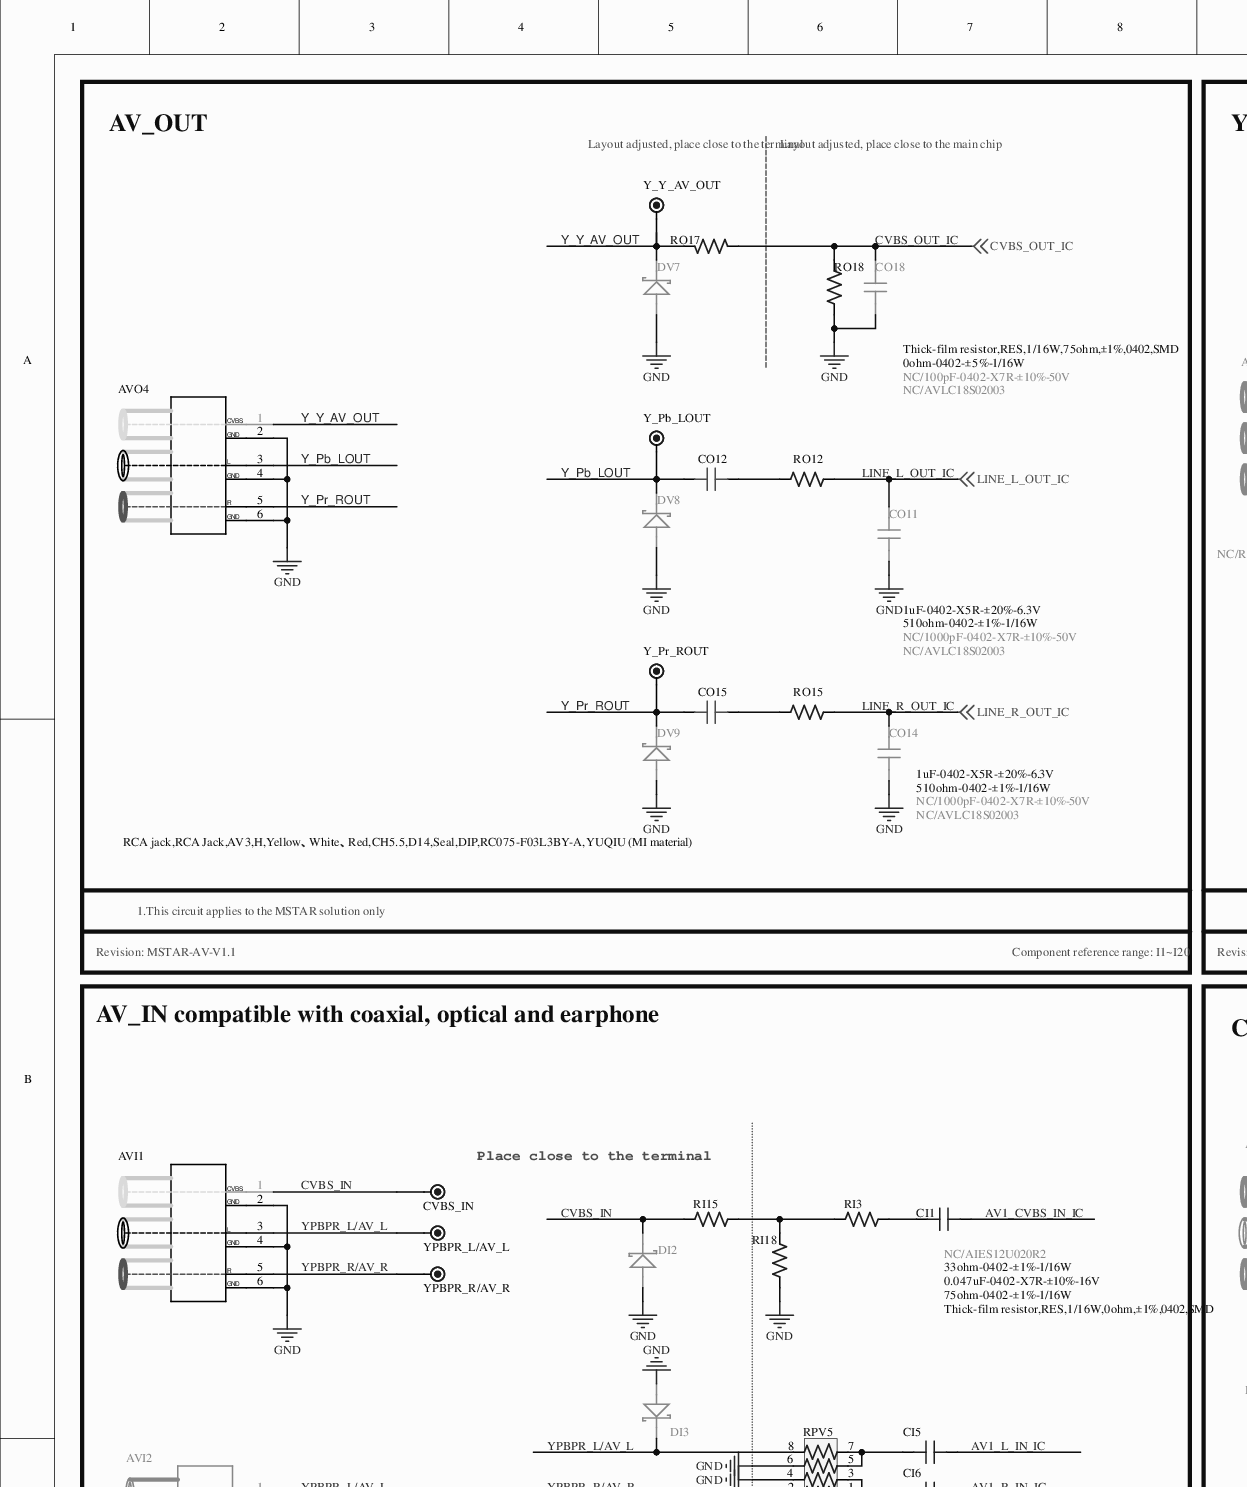
[diagram p0: MISC116569-10.SchDoc, top left]
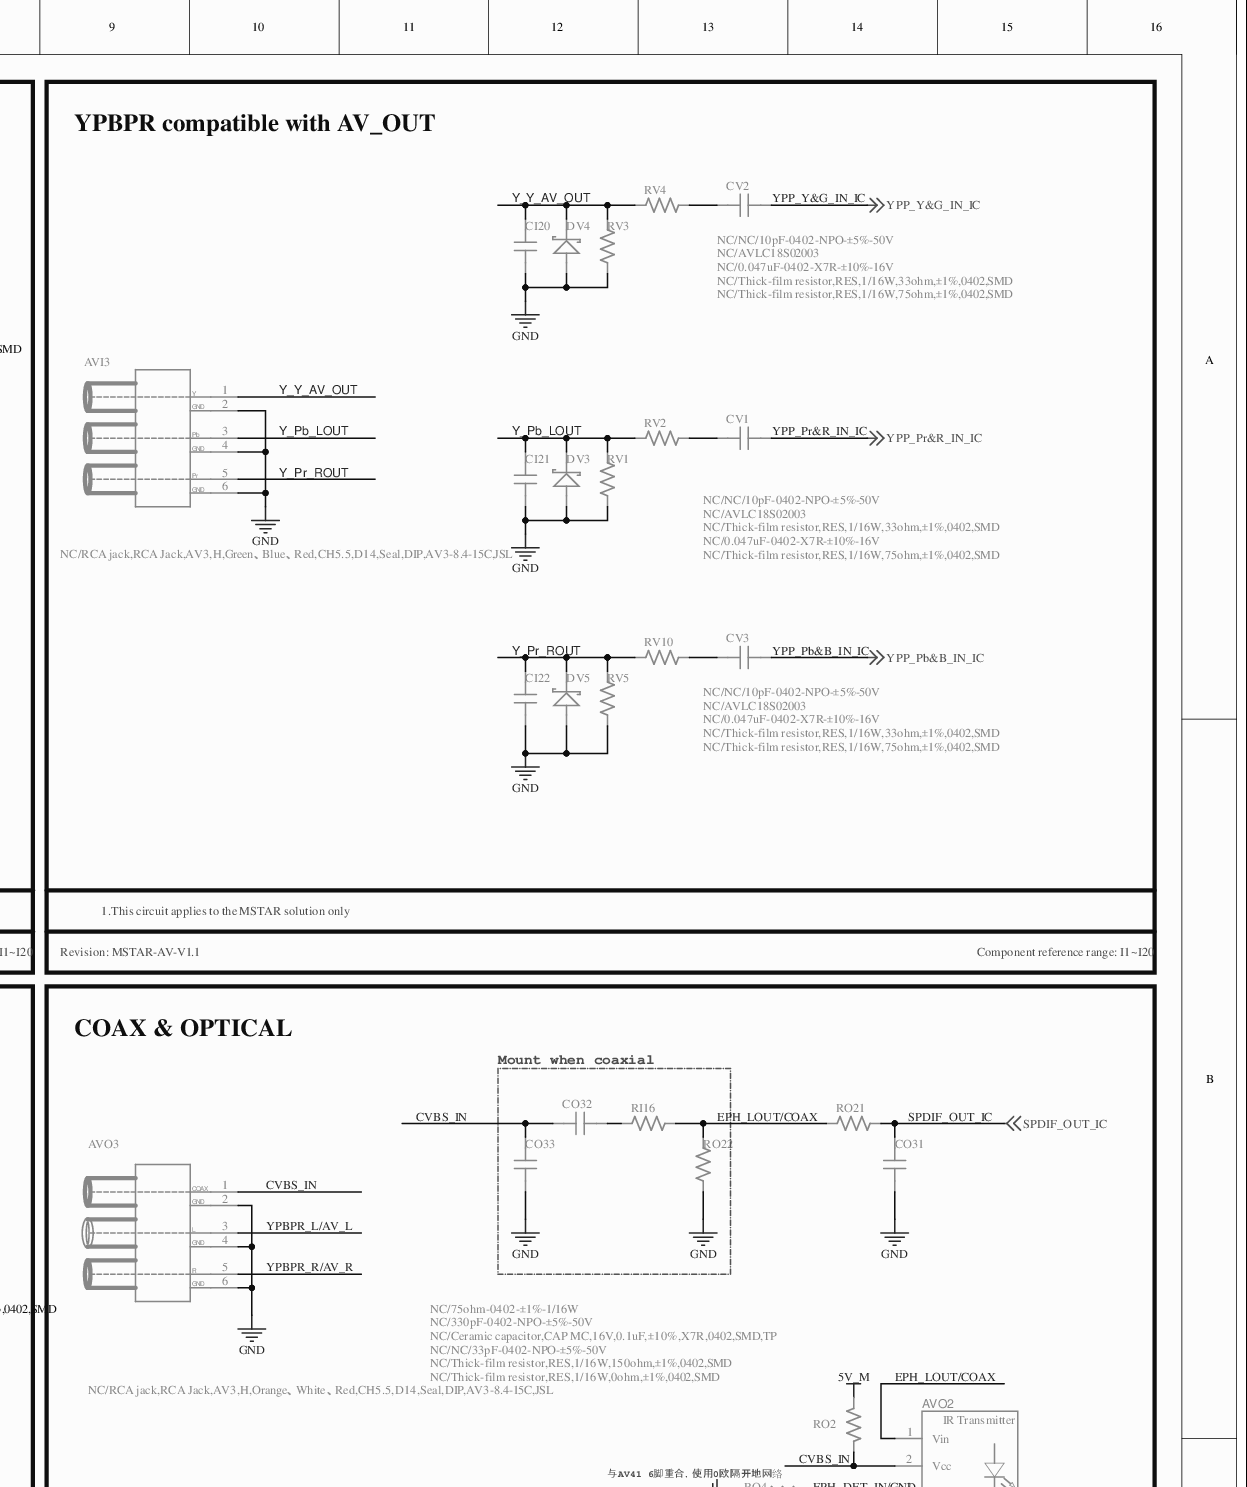
[diagram p1: MISC116569-10.SchDoc, top right]
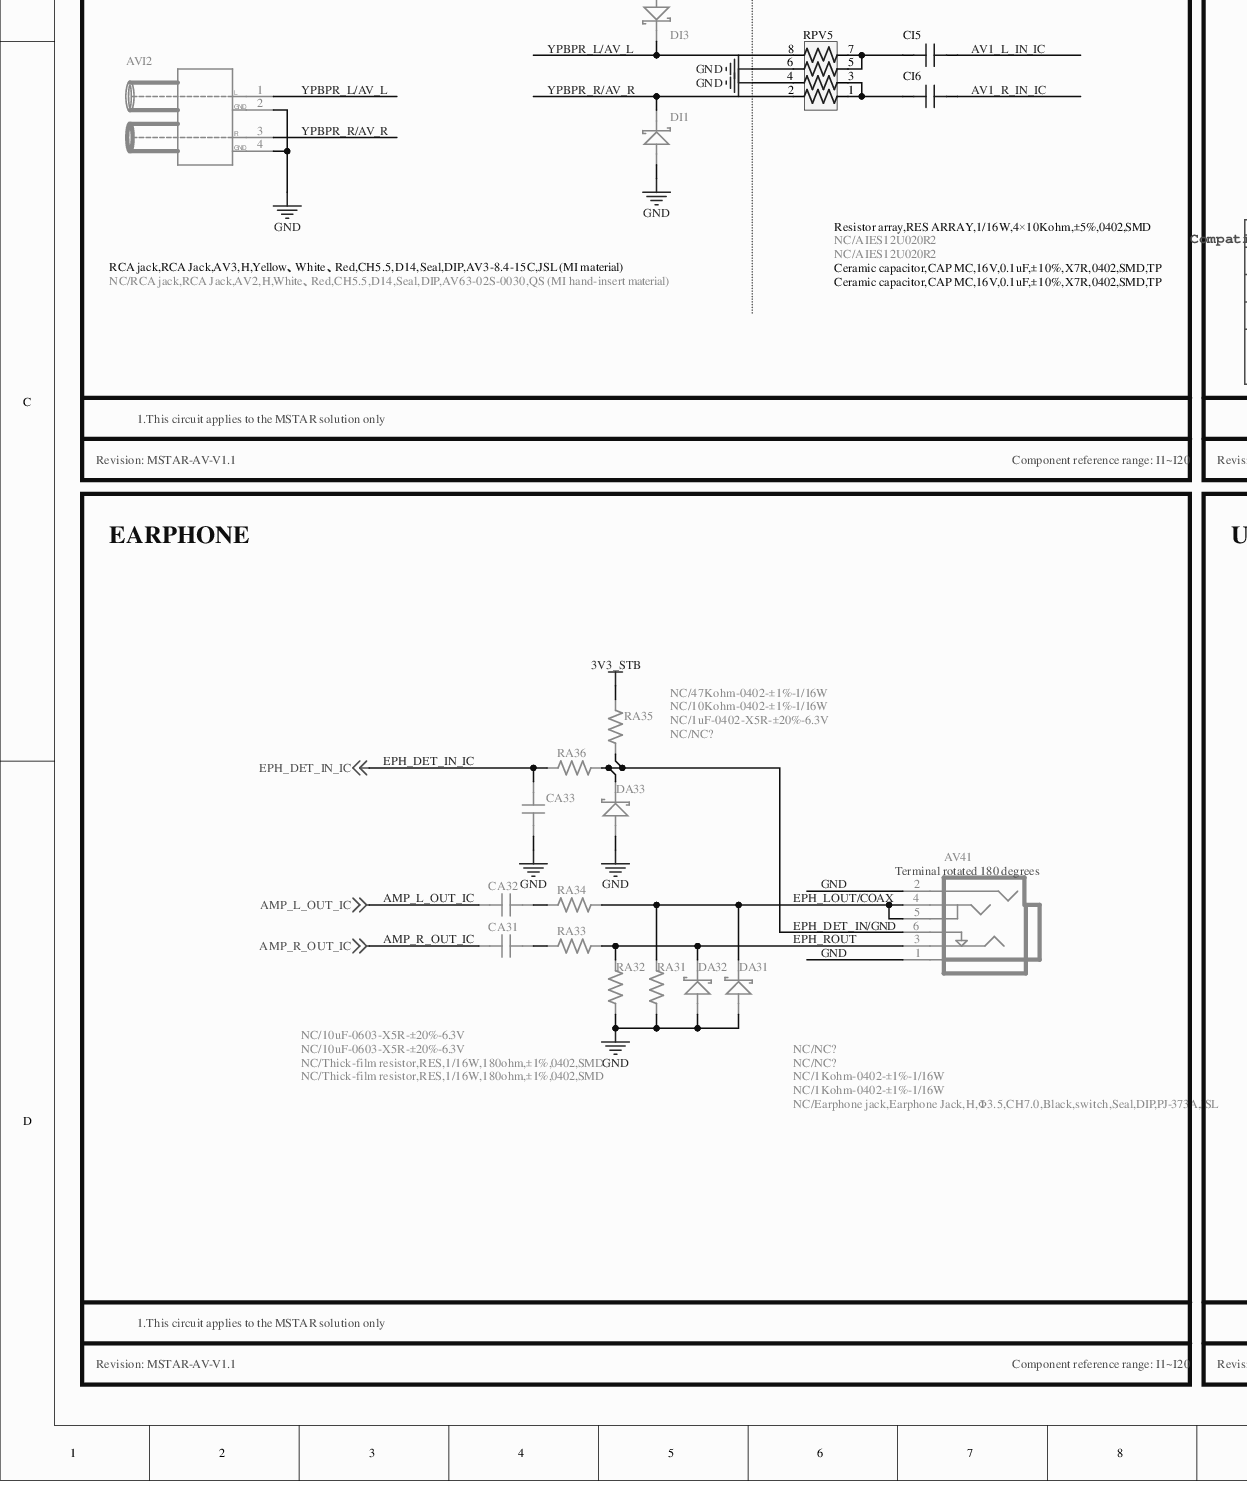
[diagram p2: MISC116569-10.SchDoc, bottom left]
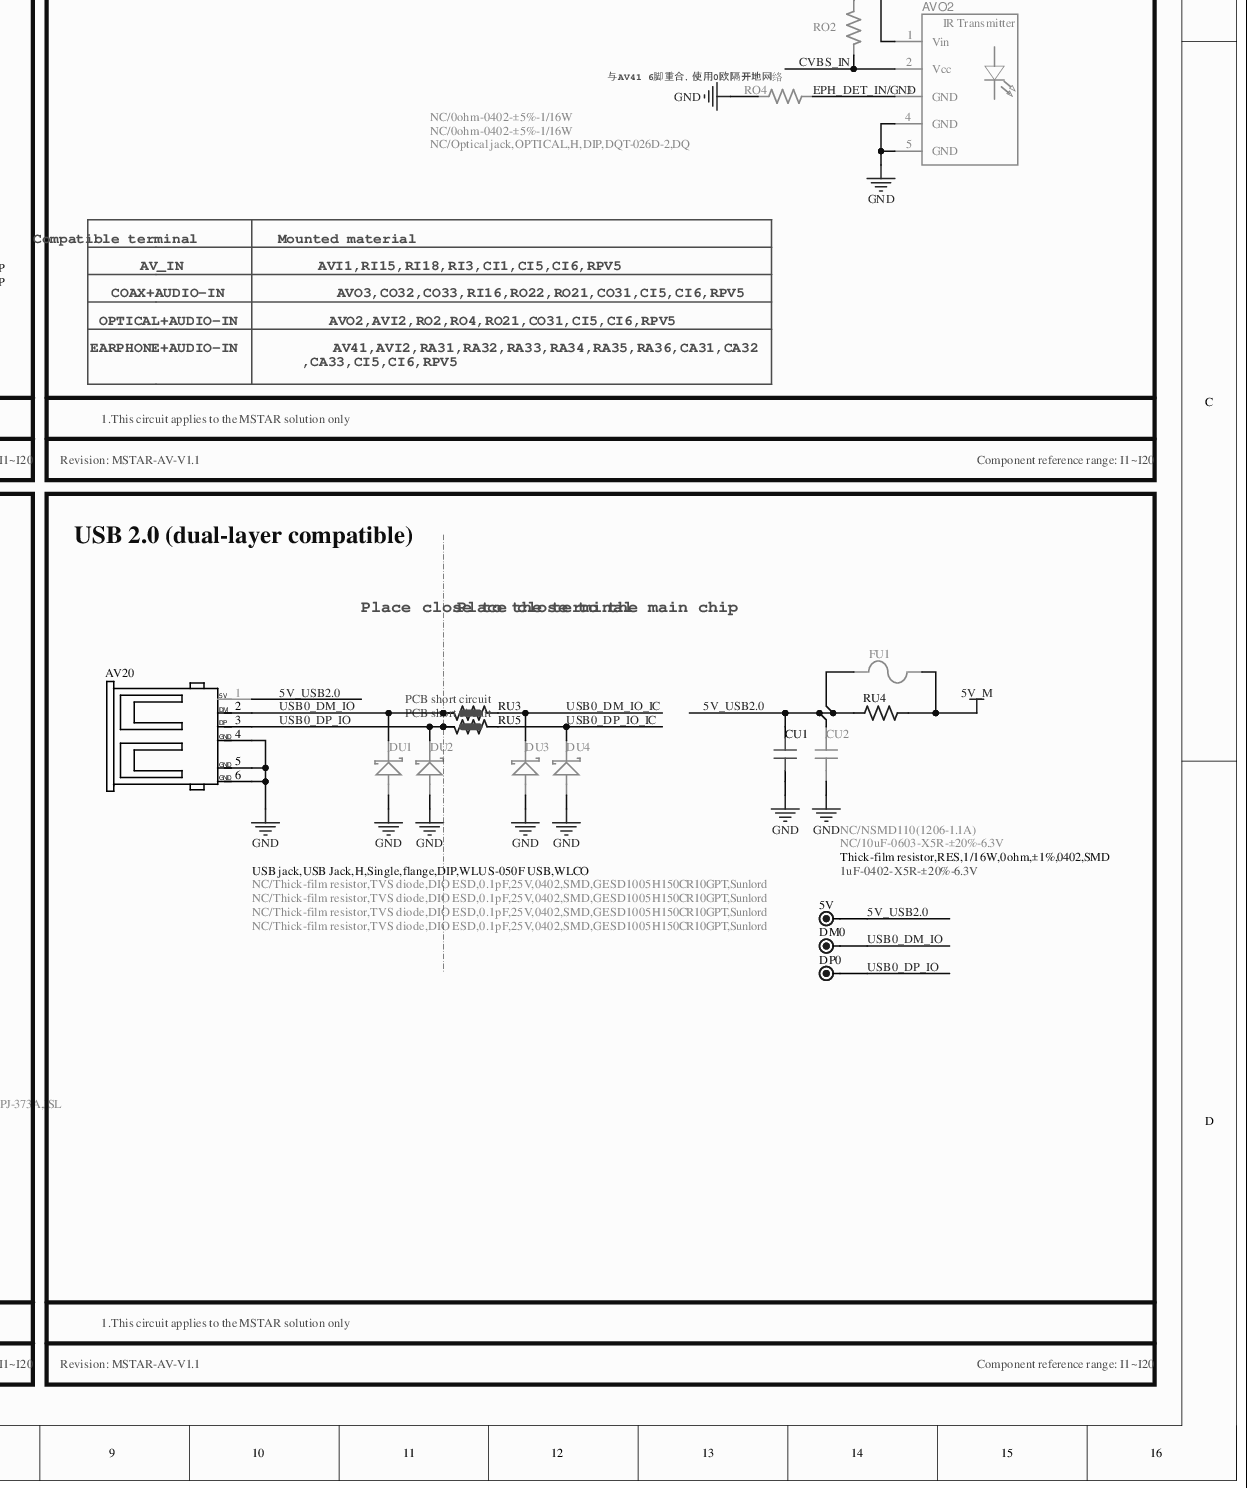
[diagram p3: MISC116569-10.SchDoc, bottom right]
# Altium project MISC116569-15.PrjPCB (part 5 of 8)

## Sheet MISC116569-10.SchDoc
size 444 x 533 mm

### Parts
5V  DM0  [TP]  (value not drawn)
AV20  USB jack,USB Jack,H,Single,flange,DIP,WLUS-050F USB,WLCO  [USB1-HD-2]
AV41  NC/Earphone jack,Earphone Jack,H,Φ3.5,CH7.0,Black,switch,Seal,DIP,PJ-373A,JSL  [PHONE-HD-42]
AVI1  RCA jack,RCA Jack,AV3,H,Yellow、White、Red,CH5.5,D14,Seal,DIP,AV3-8.4-15C,JSL (MI material)  [AV3-H14-15]
AVI2  NC/RCA jack,RCA Jack,AV2,H,White、Red,CH5.5,D14,Seal,DIP,AV63-02S-0030,QS (MI hand-insert material)  [AV2-H14-15]
AVI3  NC/RCA jack,RCA Jack,AV3,H,Green、Blue、Red,CH5.5,D14,Seal,DIP,AV3-8.4-15C,JSL  [AV3-H14-15]
AVO2  NC/Optical jack,OPTICAL,H,DIP,DQT-026D-2,DQ  [OPTICAL-HD-3]
AVO3  NC/RCA jack,RCA Jack,AV3,H,Orange、White、Red,CH5.5,D14,Seal,DIP,AV3-8.4-15C,JSL  [AV3-H14-15]
AVO4  RCA jack,RCA Jack,AV3,H,Yellow、White、Red,CH5.5,D14,Seal,DIP,RC075-F03L3BY-A,YUQIU (MI material)  [AV3-H14-15]
CA31  NC/10uF-0603-X5R-±20%-6.3V  [C0603]
CA32  NC/10uF-0603-X5R-±20%-6.3V  [C0603]
CA33  NC/1uF-0402-X5R-±20%-6.3V  [C0402]
CI1  0.047uF-0402-X7R-±10%-16V  [C0402]
CI5  Ceramic capacitor,CAP MC,16V,0.1uF,±10%,X7R,0402,SMD,TP  [C0402]
CI6  Ceramic capacitor,CAP MC,16V,0.1uF,±10%,X7R,0402,SMD,TP  [C0402]
CI20  NC/NC/10pF-0402-NPO-±5%-50V  [C0402]
CI21  NC/NC/10pF-0402-NPO-±5%-50V  [C0402]
CI22  NC/NC/10pF-0402-NPO-±5%-50V  [C0402]
CO11  NC/1000pF-0402-X7R-±10%-50V  [C0402]
CO12  1uF-0402-X5R-±20%-6.3V  [C0402]
CO14  NC/1000pF-0402-X7R-±10%-50V  [C0402]
CO15  1uF-0402-X5R-±20%-6.3V  [C0402]
CO18  NC/100pF-0402-X7R-±10%-50V  [C0402]
CO31  NC/NC/33pF-0402-NPO-±5%-50V  [C0402]
CO32  NC/Ceramic capacitor,CAP MC,16V,0.1uF,±10%,X7R,0402,SMD,TP  [C0402]
CO33  NC/330pF-0402-NPO-±5%-50V  [C0402]
CU1  1uF-0402-X5R-±20%-6.3V  [C0402]
CU2  NC/10uF-0603-X5R-±20%-6.3V  [C0603]
CV1  NC/0.047uF-0402-X7R-±10%-16V  [C0402]
CV2  NC/0.047uF-0402-X7R-±10%-16V  [C0402]
CV3  NC/0.047uF-0402-X7R-±10%-16V  [C0402]
CVBS_IN  DM0  [TP]  (value not drawn)
DA31  NC/NC?  [DIODE-S0402]
DA32  NC/NC?  [DIODE-S0402]
DA33  NC/NC?  [DIODE-S0402]
DI1  NC/AIES12U020R2  [DIODE-S0402]
DI2  NC/AIES12U020R2  [DIODE-S0402]
DI3  NC/AIES12U020R2  [DIODE-S0402]
DM0  DM0  [TP]  (value not drawn)
DP0  DM0  [TP]  (value not drawn)
DU1  NC/Thick-film resistor,TVS diode,DIO ESD,0.1pF,25V,0402,SMD,GESD1005H150CR10GPT,Sunlord  [DIODE-S0402]
DU2  NC/Thick-film resistor,TVS diode,DIO ESD,0.1pF,25V,0402,SMD,GESD1005H150CR10GPT,Sunlord  [DIODE-S0402]
DU3  NC/Thick-film resistor,TVS diode,DIO ESD,0.1pF,25V,0402,SMD,GESD1005H150CR10GPT,Sunlord  [DIODE-S0402]
DU4  NC/Thick-film resistor,TVS diode,DIO ESD,0.1pF,25V,0402,SMD,GESD1005H150CR10GPT,Sunlord  [DIODE-S0402]
DV3  NC/AVLC18S02003  [DIODE-S0402]
DV4  NC/AVLC18S02003  [DIODE-S0402]
DV5  NC/AVLC18S02003  [DIODE-S0402]
DV7  NC/AVLC18S02003  [DIODE-S0402]
DV8  NC/AVLC18S02003  [DIODE-S0402]
DV9  NC/AVLC18S02003  [DIODE-S0402]
FU1  NC/NSMD110(1206-1.1A)  [FUSE1.1A-S]
RA31  NC/1Kohm-0402-±1%-1/16W  [R0402]
RA32  NC/1Kohm-0402-±1%-1/16W  [R0402]
RA33  NC/Thick-film resistor,RES,1/16W,180ohm,±1%,0402,SMD  [R0402]
RA34  NC/Thick-film resistor,RES,1/16W,180ohm,±1%,0402,SMD  [R0402]
RA35  NC/47Kohm-0402-±1%-1/16W  [R0402]
RA36  NC/10Kohm-0402-±1%-1/16W  [R0402]
RI3  33ohm-0402-±1%-1/16W  [R0402]
RI15  Thick-film resistor,RES,1/16W,0ohm,±1%,0402,SMD  [R0402]
RI16  NC/Thick-film resistor,RES,1/16W,0ohm,±1%,0402,SMD  [R0402]
RI18  75ohm-0402-±1%-1/16W  [R0402]
RO2  NC/0ohm-0402-±5%-1/16W  [R0402]
RO4  NC/0ohm-0402-±5%-1/16W  [R0402]
RO12  510ohm-0402-±1%-1/16W  [R0402]
RO15  510ohm-0402-±1%-1/16W  [R0402]
RO17  0ohm-0402-±5%-1/16W  [R0402]
RO18  Thick-film resistor,RES,1/16W,75ohm,±1%,0402,SMD  [R0402]
RO21  NC/Thick-film resistor,RES,1/16W,150ohm,±1%,0402,SMD  [R0402]
RO22  NC/75ohm-0402-±1%-1/16W  [R0402]
RPV5  Resistor array,RES ARRAY,1/16W,4×10Kohm,±5%,0402,SMD  [RA0402]
RU3  NC/0ohm-0402-PCB  [R0402SC]  (value not drawn)
RU4  Thick-film resistor,RES,1/16W,0ohm,±1%,0402,SMD  [R0402]
RU5  NC/0ohm-0402-PCB  [R0402SC]  (value not drawn)
RV1  NC/Thick-film resistor,RES,1/16W,75ohm,±1%,0402,SMD  [R0402]
RV2  NC/Thick-film resistor,RES,1/16W,33ohm,±1%,0402,SMD  [R0402]
RV3  NC/Thick-film resistor,RES,1/16W,75ohm,±1%,0402,SMD  [R0402]
RV4  NC/Thick-film resistor,RES,1/16W,33ohm,±1%,0402,SMD  [R0402]
RV5  NC/Thick-film resistor,RES,1/16W,75ohm,±1%,0402,SMD  [R0402]
RV10  NC/Thick-film resistor,RES,1/16W,33ohm,±1%,0402,SMD  [R0402]
Y_Pb_LOUT  DM0  [TP]  (value not drawn)
Y_Pr_ROUT  DM0  [TP]  (value not drawn)
Y_Y_AV_OUT  DM0  [TP]  (value not drawn)
YPBPR_L/AV_L  DM0  [TP]  (value not drawn)
YPBPR_R/AV_R  DM0  [TP]  (value not drawn)

### Blocks framed on the sheet
AV_OUT: AVO4 CO11 CO12 CO14 CO15 CO18 DV7-DV9 RO12 RO15 RO17 RO18 Y_Pb_LOUT Y_Pr_ROUT Y_Y_AV_OUT
YPBPR compatible with AV_OUT: AVI3 CI20-CI22 CV1-CV3 DV3-DV5 RV1-RV5 RV10
AV_IN compatible with coaxial, optical and earphone: AVI1 AVI2 CI1 CI5 CI6 CVBS_IN DI1-DI3 RI3 RI15 RI18 RPV5 YPBPR_L/AV_L YPBPR_R/AV_R
COAX & OPTICAL: AVO2 AVO3 CO31 RO2 RO4 RO21
Mount when coaxial: CO32 CO33 RI16 RO22
EARPHONE: AV41 CA31-CA33 DA31-DA33 RA31-RA36
USB 2.0 (dual-layer compatible): 5V AV20 CU1 CU2 DM0 DP0 DU1-DU4 FU1 RU3-RU5

### Nets
3V3_STB: RA35.2
5V_M: FU1.2 RO2.1 RU4.2
GND: AV20.4 AV20.5 AV20.6 AV41.1 AV41.2 AVI1.2(GND) AVI1.4 AVI1.6 AVI2.2 AVI2.4 AVI3.2(CVBS) AVI3.4(Rin) AVI3.6(Lin) AVO2.4(GND) AVO2.5(GND) AVO3.2(GND) AVO3.4(GND) AVO3.6(GND) AVO4.2(GND) AVO4.4 AVO4.6 CA33.1 CI20.2 CI21.2 CI22.2 CO11.1 CO14.1 CO18.1 CO31.1 CO33.1 CU1.2 CU2.2 DA31.A DA32.A DA33.A DI1.A DI2.A DI3.A DU1.A DU2.A DU3.A DU4.A DV3.A DV4.A DV5.A DV7.A DV8.A DV9.A RA31.1 RA32.1 RI18.1 RO4.1 RO18.1 RO22.1 RPV5.4 RPV5.6 RV1.1 RV3.1 RV5.1
5V_USB2.0: 5V.1 AV20.1 CU1.1 CU2.1 FU1.1 RU4.1
AMP_L_OUT_IC: CA32.2 ; off-sheet AMP_L_OUT_IC
AMP_R_OUT_IC: CA31.2 ; off-sheet AMP_R_OUT_IC
AV1_CVBS_IN_IC: CI1.1
AV1_L_IN_IC: CI5.1
AV1_R_IN_IC: CI6.1
CVBS_IN: AVI1.1(R) AVO2.2(Vcc) AVO3.1(R) CO32.2 CO33.2 CVBS_IN.1 DI2.K RI15.1 RO2.2
CVBS_OUT_IC: CO18.2 RO17.1 RO18.2 ; off-sheet CVBS_OUT_IC
EPH_DET_IN/GND: AV41.6 AVO2.3(GND) DA33.K RA35.1 RA36.2 RO4.2
EPH_DET_IN_IC: CA33.2 RA36.1 ; off-sheet EPH_DET_IN_IC
EPH_LOUT/COAX: AV41.4 AV41.5 AVO2.1(Vin) DA31.K RA31.2 RA34.2 RI16.2 RO21.1 RO22.2
EPH_ROUT: AV41.3 DA32.K RA32.2 RA33.2
LINE_L_OUT_IC: CO11.2 RO12.1 ; off-sheet LINE_L_OUT_IC
LINE_R_OUT_IC: CO14.2 RO15.1 ; off-sheet LINE_R_OUT_IC
SPDIF_OUT_IC: CO31.2 RO21.2 ; off-sheet SPDIF_OUT_IC
USB0_DM_IO: AV20.2 DM0.1 DU1.K RU3.2 RU3.3
USB0_DM_IO_IC: DU3.K RU3.1
USB0_DP_IO: AV20.3 DP0.1 DU2.K RU5.2 RU5.3
USB0_DP_IO_IC: DU4.K RU5.1
Y_Pb_LOUT: AVI3.3(GND) AVO4.3 CI21.1 CO12.2 DV3.K DV8.K RV1.2 RV2.1 Y_Pb_LOUT.1
Y_Pr_ROUT: AVI3.5(GND) AVO4.5 CI22.1 CO15.2 DV5.K DV9.K RV5.2 RV10.1 Y_Pr_ROUT.1
Y_Y_AV_OUT: AVI3.1(GND) AVO4.1(R) CI20.1 DV4.K DV7.K RO17.2 RV3.2 RV4.1 Y_Y_AV_OUT.1
YPBPR_L/AV_L: AVI1.3 AVI2.1(R) AVO3.3(L) DI3.K RPV5.8 YPBPR_L/AV_L.1
YPBPR_R/AV_R: AVI1.5 AVI2.3 AVO3.5(R) DI1.K RPV5.2 YPBPR_R/AV_R.1
YPP_Pb&B_IN_IC: CV3.2 ; off-sheet YPP_Pb&B_IN_IC
YPP_Pr&R_IN_IC: CV1.2 ; off-sheet YPP_Pr&R_IN_IC
YPP_Y&G_IN_IC: CV2.2 ; off-sheet YPP_Y&G_IN_IC
NetCA31_1: CA31.1 RA33.1
NetCA32_1: CA32.1 RA34.1
NetCI1_2: CI1.2 RI3.2
NetCI5_2: CI5.2 RPV5.5 RPV5.7
NetCI6_2: CI6.2 RPV5.1 RPV5.3
NetCO12_1: CO12.1 RO12.2
NetCO15_1: CO15.1 RO15.2
NetCO32_1: CO32.1 RI16.1
NetCV1_1: CV1.1 RV2.2
NetCV2_1: CV2.1 RV4.2
NetCV3_1: CV3.1 RV10.2
NetRI3_1: RI3.1 RI15.2 RI18.2

### Notes on the sheet
- Layout adjusted, place close to the terminal
- Layout adjusted, place close to the main chip
- 1.This circuit applies to the MSTAR solution only
- Revision: MSTAR-AV-V1.1
- Component reference range: I1~I20
- Place close to the terminal
- 与AV41 6脚重合，使用0欧隔开地网络
- AV_IN
- Compatible terminal
- Mounted material
- AVI1,RI15,RI18,RI3,CI1,CI5,CI6,RPV5
- COAX+AUDIO-IN
- OPTICAL+AUDIO-IN
- AVO2,AVI2,RO2,RO4,RO21,CO31,CI5,CI6,RPV5
- AVO3,CO32,CO33,RI16,RO22,RO21,CO31,CI5,CI6,RPV5
- EARPHONE+AUDIO-IN
- ,CA33,CI5,CI6,RPV5
- AV41,AVI2,RA31,RA32,RA33,RA34,RA35,RA36,CA31,CA32
- Place close to the main chip
- (near AV41) Terminal rotated 180 degrees

### Library data of the parts
5V CVBS_IN DM0 DP0 Y_Pb_LOUT Y_Pr_ROUT Y_Y_AV_OUT YPBPR_L/AV_L YPBPR_R/AV_R = TEST
AV20 = XXX.XXX.0002687: USB jack,USB Jack,H,Single,flange,DIP,103411271,VAST-DLMI
AV41 = XXX.XXX.0002138: Earphone jack,Earphone Jack,H,Φ3.5,CH7.0,Black,switch,Seal,DIP,PJ7724-F05L3BY-D,YUQIU-DLMI
AVI1 AVO4 = RCA端子,RCA Jack,AV3,H,Yellow、White、Red,CH5.5,D14,Seal,DIP,RC075-F03L3BY-A,YUQIU-DLMI-AV: CN-AV-D14-#-#
AVI2 = RCA端子,RCA Jack,AV2,H,White、Red,CH5.5,D14,Seal,DIP,AV63-02S-0030,QS(MI手插物料)-DLMI-AUDIO: CN-AUDIO-D14-#-#
AVI3 = RCA端子,RCA Jack,AV3,H,Green、Blue、Red,CH5.5,D14,Seal,DIP,RC075-F03L3BY-B,YUQIU-DLMI-YPbPr: CN-YPbPr-D14-#-#
AVO2 = GQ-03-08-DLMI: CN-DLMI-optical fiber
AVO3 = RCA端子,RCA Jack,AV3,H,Orange、White、Red,CH5.5,D14,Seal,DIP,RC075-F03L3BY-C,YUQIU-DLMI
CA31 CA32 = 004.003.0000383-D: Ceramic capacitor,CAP MC,6.3V,10uF,±20%,X5R,0603,SMD,TP-D
CA33 CO12 CO15 = 004.003.0000361-D: Ceramic capacitor,CAP MC,6.3V,0.47uF,±10%,X5R,0402,SMD,TP-D
CI1 CV1-CV3 = 0.047uF-0402-X7R-±10%-16V-D
CI5 CI6 = 0.1uF-0402-Y5V-+80%-20%-16V-D
CI20-CI22 = 10pF-0402-NPO-±5%-50V-D
CO11 CO14 CO18 = 1000pF-0402-X7R-±10%-50V-D
CO31 = 33pF-0402-NPO-±5%-50V-D
CO32 = 004.003.0000403-D: Ceramic capacitor,CAP MC,16V,0.1uF,±20%,X5R,0402,SMD,TP-D
CO33 = 330pF-0402-NPO-±5%-50V-D
CU1 = 1uF-0402-X5R-±20%-6.3V-D
CU2 = 10uF-0603-X5R-±20%-6.3V-D
DA31-DA33 DV3-DV5 DV7-DV9 = AVLC18S02003-D
DI1-DI3 = AIES12U020R2-D
DU1-DU4 = 004.005.0000203-D: TVS diode,DIO ESD,0.2pF,25V,0402,SMD,AIES12U020R2,AMOTECH-D
FU1 = 004.026.0000039-D: Resettable fuse,FUSE PTC,1.1A,6V,1206,SMD,TP,TLC-D
RA31 RA32 = 1Kohm-0402-±5%-1/16W-D
RA33 RA34 RO21 = 004.002.0000609-D: Thick-film resistor,RES,1/16W,180ohm,±5%,0402,SMD-D
RA35 = 47Kohm-0402-±5%-1/16W-D
RA36 = 10Kohm-0402-±5%-1/16W-D
RI3 RO4 RV2 RV4 RV10 = 33ohm-0402-±5%-1/16W-D
RI15 RI16 RO17 RU4 = 004.002.0000558-D: Thick-film resistor,RES,1/16W,0ohm,±5%,0402,SMD-D
RI18 RO18 RV1 RV3 RV5 = 75ohm-0402-±5%-1/16W-D
RO2 = 0ohm-0402-±5%-1/16W-D
RO12 RO15 = 510ohm-0402-±5%-1/16W-D
RO22 = 004.002.0000568-D: Thick-film resistor,RES,1/16W,100ohm,±5%,0402,SMD-D
RPV5 = 4*100ohm-0402-±5%-1/16W-D
RU3 RU5 = 0ohm-0402-PCB-D